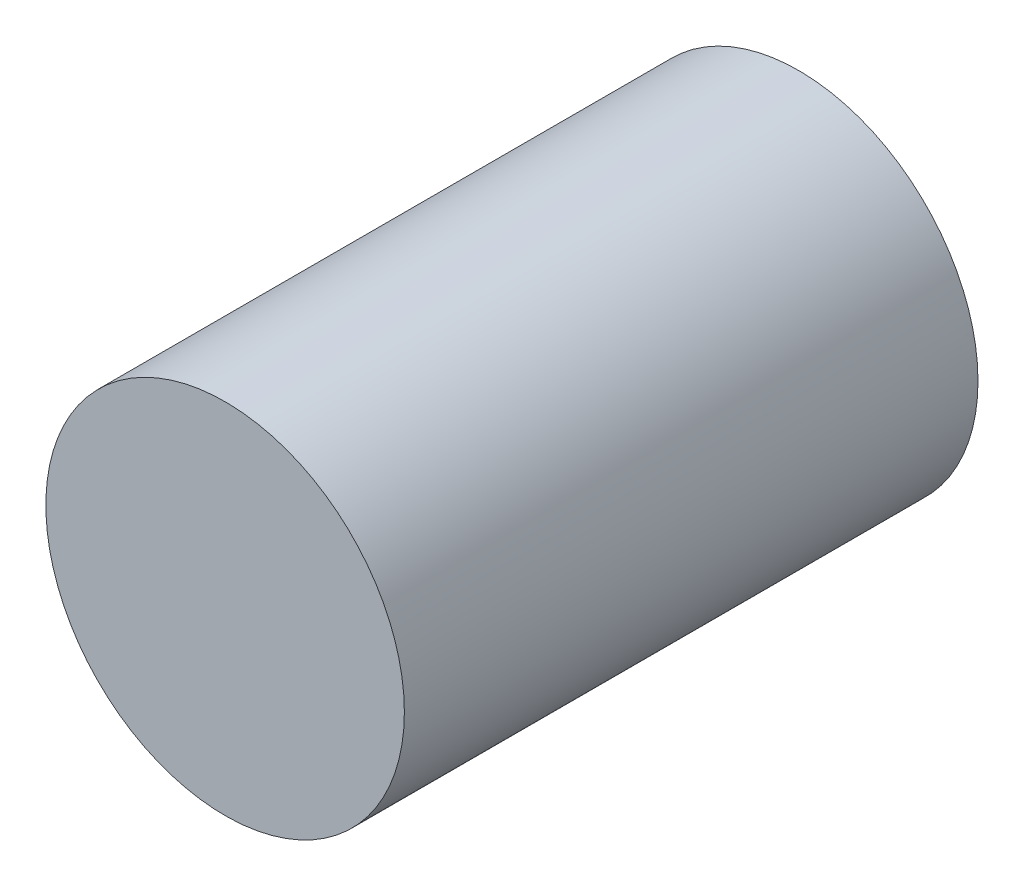
from build123d import *

# Parameters (mm, degrees)
SKETCH_1_R      = 25
EXTRUDE_1_DEPTH = 80


with BuildPart() as part:
    # 草图1 → 凸台-拉伸1 (new body)
    with BuildSketch(Plane.XY):
        Circle(SKETCH_1_R)
    extrude(amount=-EXTRUDE_1_DEPTH)


solid = part.part
